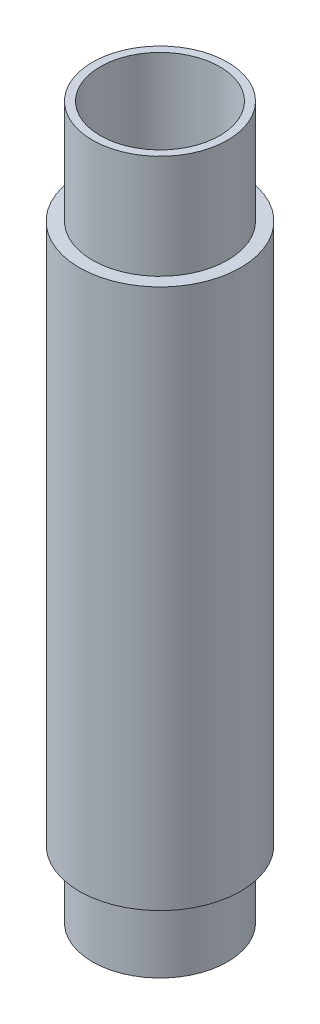
from build123d import *


with BuildPart() as part:
    # 草图1 → 旋转1 (revolve)
    with BuildSketch(Plane.XY, mode=Mode.PRIVATE) as revolve_1_sk:
        Polygon((57.5, 470.011904762), (57.5, -214.618095238), (65, -214.618095238), (65, -149.618095238), (77.5, -149.618095238), (77.5, 370.011904762), (65, 370.011904762), (65, 470.011904762), align=None)
    revolve(revolve_1_sk.sketch.rotate(Axis((0, 125.678571429, 0), (0, -1, 0)), 90), axis=Axis((0, 125.678571429, 0), (0, -1, 0)))


solid = part.part
